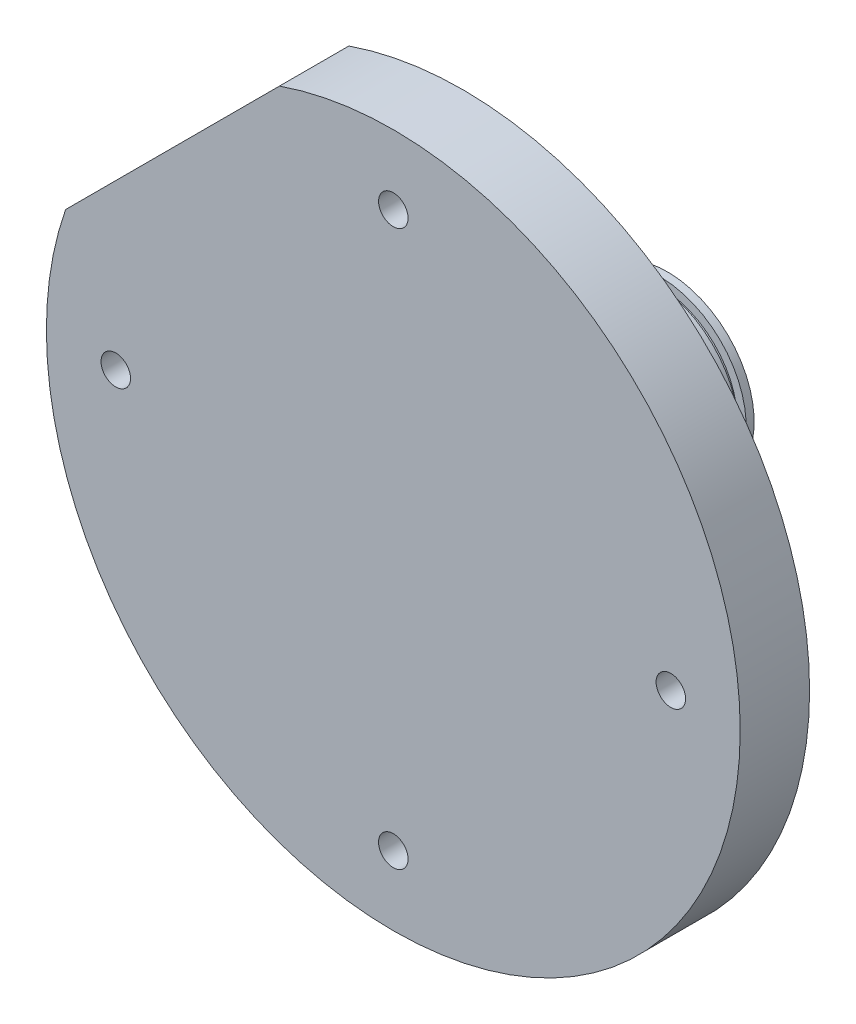
from build123d import *

# Parameters (mm, degrees)
SKETCH_4_OUTSIDE_W       = 260.734
SKETCH_4_OUTSIDE_H       = 260.734
SKETCH_4_OUTSIDE_R       = 22.5
CUT_EXTRUDE_2_DEPTH      = 2.2
HOLE_WIZARD_M10_1_D      = 8.5
PATTERN_CIRCULAR_1_COUNT = 4
CUT_EXTRUDE_5_DEPTH      = 154.242815166
HOLE_WIZARD_M10_2_D      = 8.5
HOLE_WIZARD_M10_2_DEPTH  = 60
HOLE_WIZARD_M10_2_TIP    = 2.553657631


with BuildPart() as part:
    # 草图1 → 旋转1 (revolve)
    with BuildSketch(Plane(origin=(0, 0, 0), x_dir=(1, 0, 0), z_dir=(0, 1, 0))):
        Polygon((0, 0), (-100, 0), (-100, 20), (-26.5, 20), (-26.5, 49.02), (-25, 49.02), (-25, 79.02), (0, 79.02), align=None)
    revolve(axis=Axis((0, 0, 0), (0, 0, 1)))

    # 草图4 outside → 切除-拉伸2 (cut)
    with BuildSketch(Plane(origin=(0, 0, -74.52), x_dir=(-1, 0, 0), z_dir=(0, 0, -1))):
        Rectangle(SKETCH_4_OUTSIDE_W, SKETCH_4_OUTSIDE_H)
        Circle(SKETCH_4_OUTSIDE_R, mode=Mode.SUBTRACT)
    extrude(amount=CUT_EXTRUDE_2_DEPTH, mode=Mode.SUBTRACT)

    # M10 螺纹孔1 (through all)
    with Locations(Plane(origin=(0, 0, -20), x_dir=(-1, 0, 0), z_dir=(0, 0, -1))):
        with Locations((0, -80)):
            hole_wizard_m10_1 = Hole(HOLE_WIZARD_M10_1_D / 2)

    # 阵列(圆周)1: M10 螺纹孔1 ×4 about axis
    pattern_circular_1_axis = Axis((0, 0, 0), (0, 0, 1))
    for i in range(1, PATTERN_CIRCULAR_1_COUNT):
        add(hole_wizard_m10_1.rotate(pattern_circular_1_axis, i * 360 / PATTERN_CIRCULAR_1_COUNT), mode=Mode.SUBTRACT)

    # 草图10 → 切除-拉伸5 (cut, through all)
    with BuildSketch(Plane(origin=(0, 0, -20), x_dir=(-1, 0, 0), z_dir=(0, 0, -1))):
        Polygon((106.066017178, 21.213203436), (21.213203436, 106.066017178), (56.786089274, 141.638903017), (141.638903017, 56.786089274), align=None)
    extrude(amount=-CUT_EXTRUDE_5_DEPTH, mode=Mode.SUBTRACT)

    # M10 螺纹孔2
    with Locations(Plane(origin=(-63.639610307, 63.639610307, 0), x_dir=(0.7071067811865476, 0.7071067811865475, 0), z_dir=(-0.7071067811865475, 0.7071067811865476, 0))):
        with Locations((0, 12)):
            Hole(HOLE_WIZARD_M10_2_D / 2, depth=HOLE_WIZARD_M10_2_DEPTH)
            with Locations((0, 0, -(HOLE_WIZARD_M10_2_DEPTH + HOLE_WIZARD_M10_2_TIP / 2))):  # 118° drill point
                Cone(0, HOLE_WIZARD_M10_2_D / 2, HOLE_WIZARD_M10_2_TIP, mode=Mode.SUBTRACT)


solid = part.part
